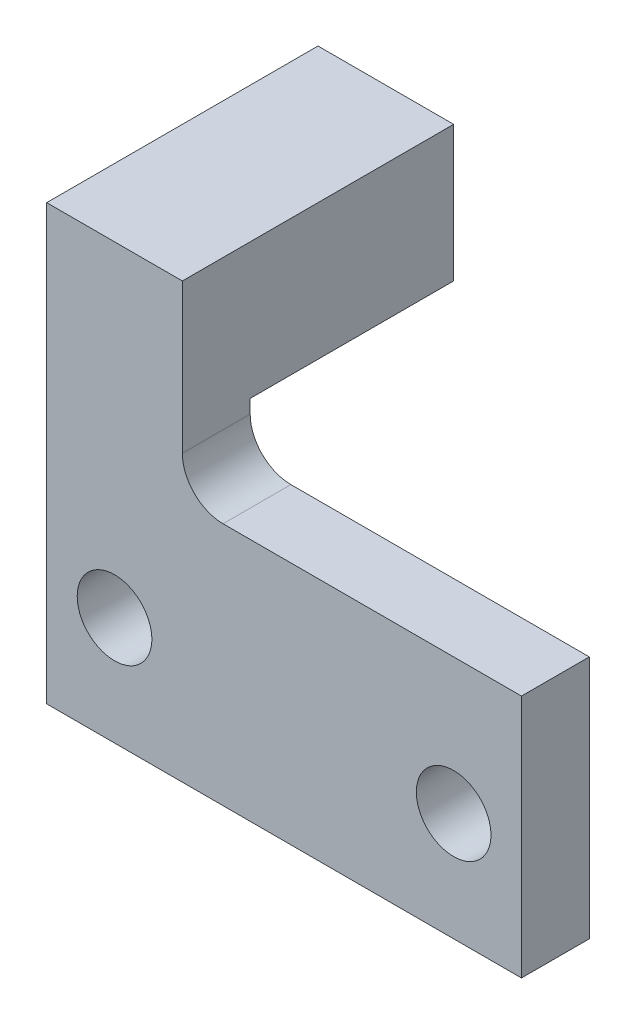
from build123d import *

# Parameters (mm, degrees)
EXTRUDE_1_DEPTH     = 5
SKETCH_3_W          = 10
SKETCH_3_H          = 10
EXTRUDE_2_DEPTH     = 20
SKETCH_4_R          = 2.75
CUT_EXTRUDE_1_DEPTH = 20


with BuildPart() as part:
    # 草图1 → 凸台-拉伸1 (new body)
    with BuildSketch(Plane.XY):
        with BuildLine():
            Line((0, 0), (35, 0))
            Line((35, 0), (35, 18))
            Line((35, 18), (13, 18))
            ThreePointArc((13, 18), (10.878679656, 18.878679656), (10, 21))
            Line((10, 21), (10, 22))
            Line((10, 22), (0, 22))
            Line((0, 22), (0, 0))
        make_face()
    extrude(amount=EXTRUDE_1_DEPTH)

    # 草图3 → 凸台-拉伸2 (add)
    with BuildSketch(Plane.XY.offset(5)):
        with Locations((5, 27)):
            Rectangle(SKETCH_3_W, SKETCH_3_H)
    extrude(amount=-EXTRUDE_2_DEPTH)

    # 草图4 → 切除-拉伸1 (cut)
    with BuildSketch(Plane(origin=(0, 0, 0), x_dir=(-1, 0, 0), z_dir=(0, 0, -1))):
        with Locations((-30, 8)):
            Circle(SKETCH_4_R)
        with Locations((-5, 8)):
            Circle(SKETCH_4_R)
    extrude(amount=-CUT_EXTRUDE_1_DEPTH, mode=Mode.SUBTRACT)


solid = part.part
